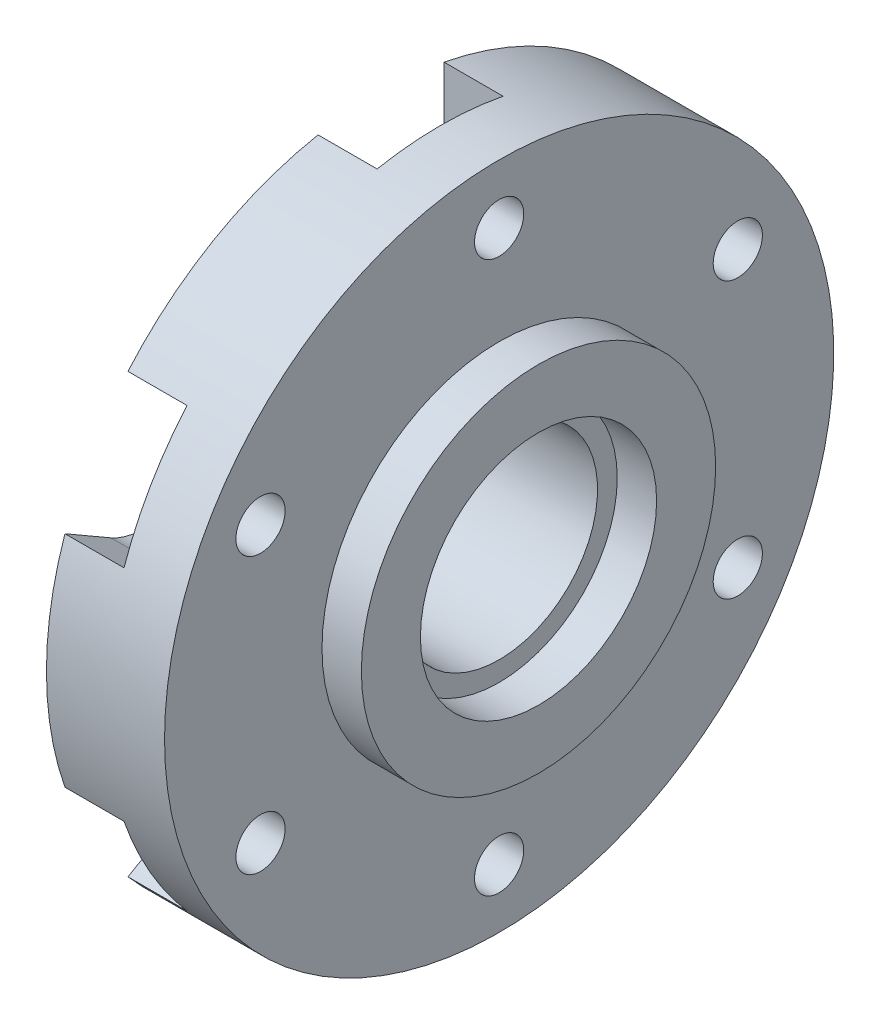
from build123d import *

# Parameters (mm, degrees)
SKETCH_2_R               = 6.25
CUT_EXTRUDE_1_DEPTH      = 127.688594593
PATTERN_CIRCULAR_1_COUNT = 6
SKETCH_3_R               = 25
CUT_EXTRUDE_2_DEPTH      = 127.688594593
CUT_EXTRUDE_START        = -15
CUT_EXTRUDE_3_DEPTH      = 15
PATTERN_CIRCULAR_2_COUNT = 6
PATTERN_CIRCULAR_3_COUNT = 6


with BuildPart() as part:
    # 草图1 → 旋转1 (revolve)
    with BuildSketch(Plane.XY, mode=Mode.PRIVATE) as revolve_1_sk:
        Polygon((0, 0), (0, 85), (30, 85), (30, 45), (40, 45), (40, 30), (30, 30), (30, 0), align=None)
    revolve(revolve_1_sk.sketch.rotate(Axis((0, 0, 0), (1, 0, 0)), 90), axis=Axis((0, 0, 0), (1, 0, 0)))

    # 草图2 → 切除-拉伸1 (cut, through all)
    with BuildSketch(Plane.ZY):
        with Locations((0, 70)):
            Circle(SKETCH_2_R)
    cut_extrude_1 = extrude(amount=-CUT_EXTRUDE_1_DEPTH, mode=Mode.SUBTRACT)

    # 阵列(圆周)1: 切除-拉伸1 ×6 about axis
    pattern_circular_1_axis = Axis((0, 0, 0), (1, 0, 0))
    for i in range(1, PATTERN_CIRCULAR_1_COUNT):
        add(cut_extrude_1.rotate(pattern_circular_1_axis, i * 360 / PATTERN_CIRCULAR_1_COUNT), mode=Mode.SUBTRACT)

    # 草图3 → 切除-拉伸2 (cut, through all)
    with BuildSketch(Plane.ZY):
        Circle(SKETCH_3_R)
    extrude(amount=-CUT_EXTRUDE_2_DEPTH, mode=Mode.SUBTRACT)

    # 草图6 → 切除-拉伸3 (cut)
    with BuildSketch(Plane.ZY.offset(CUT_EXTRUDE_START)):
        with BuildLine():
            Line((-16, 70), (-16, 83.480536654))
            ThreePointArc((-16, 83.480536654), (0, 85), (16, 83.480536654))
            Line((16, 83.480536654), (16, 70))
            ThreePointArc((16, 70), (0, 54), (-16, 70))
        make_face()
    cut_extrude_3 = extrude(amount=CUT_EXTRUDE_3_DEPTH, mode=Mode.SUBTRACT)

    # 阵列(圆周)2: 切除-拉伸3 ×6 about axis
    pattern_circular_2_axis = Axis((0, 0, 0), (1, 0, 0))
    for i in range(1, PATTERN_CIRCULAR_2_COUNT):
        add(cut_extrude_3.rotate(pattern_circular_2_axis, i * 360 / PATTERN_CIRCULAR_2_COUNT), mode=Mode.SUBTRACT)

    # 草图8 → M12 螺纹孔1 (revolve, cut)
    with BuildSketch(Plane(origin=(0, 60.621778265, 35), x_dir=(0, 0, 1), z_dir=(0, 1, 0))):
        Polygon((0, 0), (0, 21.064389157), (5.1, 18), (5.1, 0), align=None)
    hole_wizard_m12_1 = revolve(axis=Axis((-6.35, 60.621778265, 35), (1, 0, 0)), mode=Mode.SUBTRACT)

    # 阵列(圆周)3: M12 螺纹孔1 ×6 about axis
    pattern_circular_3_axis = Axis((0, 0, 0), (1, 0, 0))
    for i in range(1, PATTERN_CIRCULAR_3_COUNT):
        add(hole_wizard_m12_1.rotate(pattern_circular_3_axis, i * 360 / PATTERN_CIRCULAR_3_COUNT), mode=Mode.SUBTRACT)


solid = part.part
